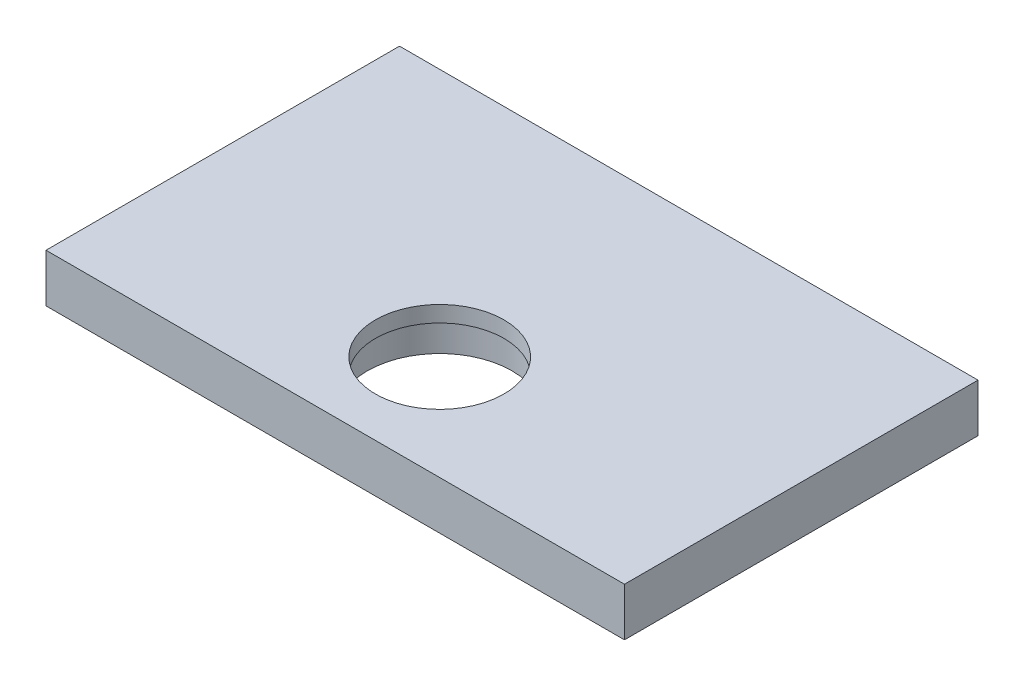
SolidWorks part; units mm, degrees
ref_plane "前视基准面" through (0, 0, 0) normal (0, 0, 1) x (1, 0, 0)
ref_plane "上视基准面" through (0, 0, 0) normal (0, 1, 0) x (1, 0, 0)
ref_plane "右视基准面" through (0, 0, 0) normal (1, 0, 0) x (0, 0, -1)
sketch "草图1" plane through (0, 0, 0) normal (0, 1, 0) x (1, 0, 0)
  line L1 (-180, -110) -> (180, -110)
  line L2 (-180, -110) -> (-180, 110)
  line L3 (-180, 110) -> (180, 110)
  line L4 (180, -110) -> (180, 110)
  line L5 (-180, -110) -> (180, 110) construction
  line L6 (-180, 110) -> (180, -110) construction
  point P0 (0, 0)
  dimension "D1" = 220
  dimension "D2" = 360
extrude "凸台-拉伸1" add sketch "草图1" along normal blind 30
sketch "草图2" plane through (0, 0, 0) normal (0, -1, 0) x (1, 0, 0)
  line L2 (180, 110) -> (180, -110) construction
  line L4 (180, -110) -> (-180, -110) construction
  circle A0 centre (0, 45) radius 40
  dimension "D1" = 80
  dimension "D2" = 155
  dimension "D3" = 180
extrude "切除-拉伸1" cut sketch "草图2" against normal through all
sketch "草图4" plane through (0, 0, 0) normal (0, -1, 0) x (1, 0, 0)
  line L0 (180, 110) -> (180, -110) construction
  line L1 (-180, 110) -> (180, 110) construction
  circle A0 centre (0, 45) radius 45
  dimension "D1" = 90
  dimension "D2" = 180
  dimension "D3" = 65
extrude "切除-拉伸3" cut sketch "草图4" against normal blind 20
